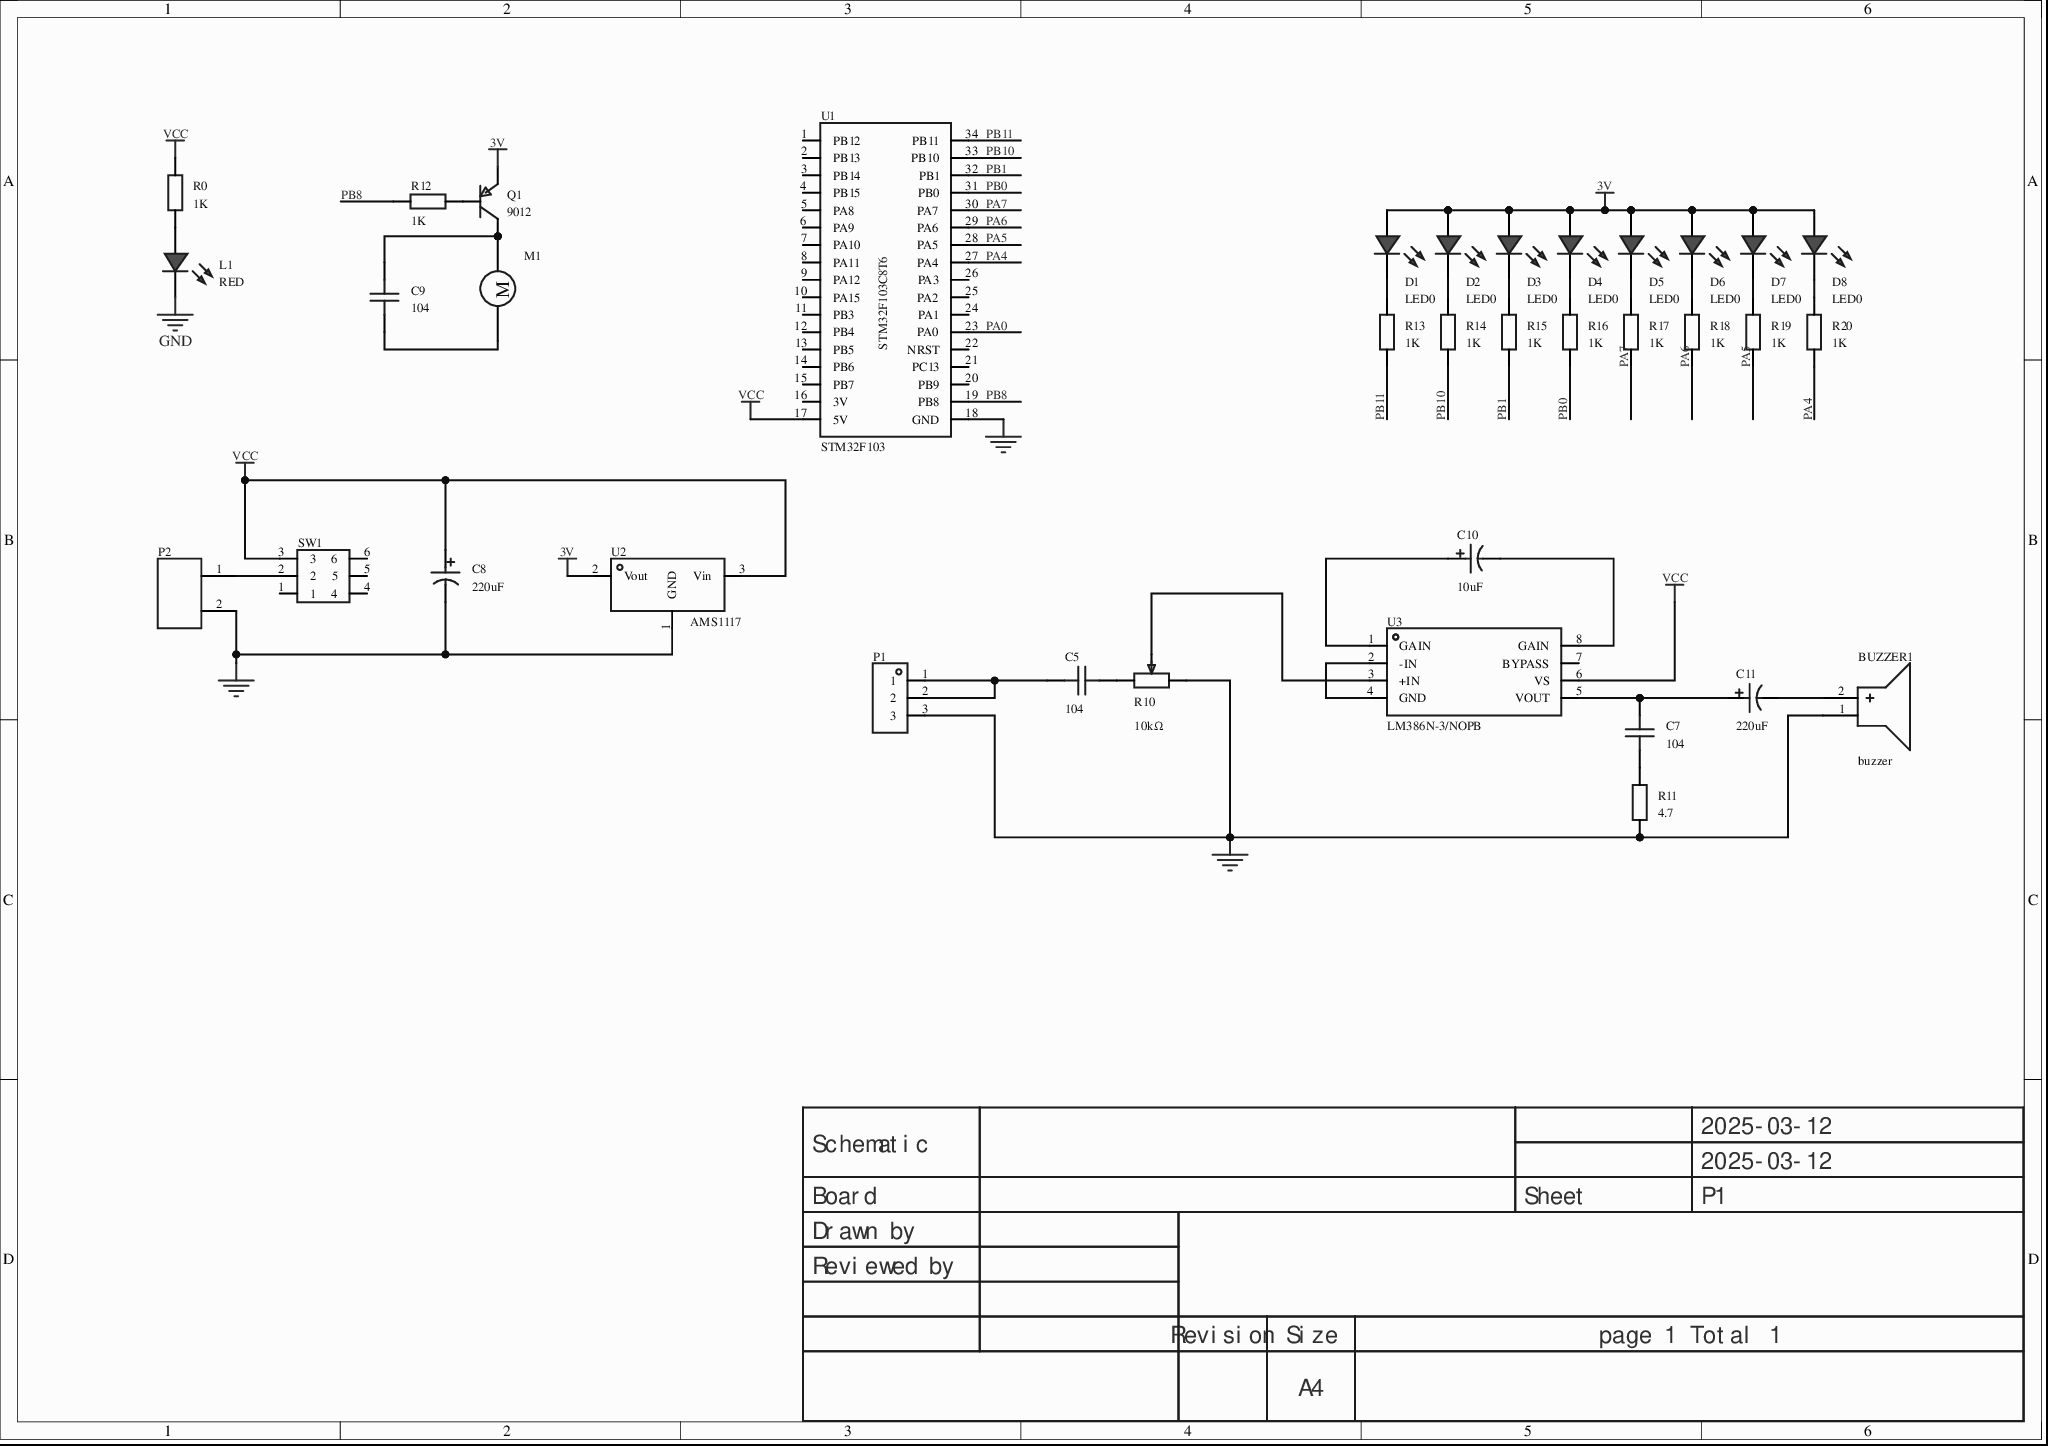
[diagram p0: MISC52120-3.schdoc]
# Altium project MISC52120-2.PrjPcb
1 sheet, 36 parts. Net scope: global (net labels, ports and power ports of the same name join across sheets).
Board file: MISC52120.pcbdoc

## Sheet MISC52120-3.schdoc
size 297 x 209 mm; Version: V1.0; @Project Name: MISC52120; @Page Count: 1; @Update Date: 2025-03-12; @Create Date: 2025-03-12; @Schematic Name: MISC52120; @Page No: 1; @Create Time: 16:08:51; @Update Time: 16:38:23; @Board Name: MISC52120

### Parts
BUZZER1  buzzer  [BUZ-TH_BD12.0-P6.00-D0.9-RD]
C5  104  [C0805]
C7  104  [C0805]
C8  220uF  [CAP-TH_BD6.3-P2.50-D1.0-FD]
C9  104  [C0805]
C10  10uF  [CAP-TH_BD5.0-P2.00-D0.8-FD]
C11  220uF  [CAP-TH_BD6.3-P2.50-D1.0-FD]
D1  LED0  [LED_TH-3mm]
D2  LED0  [LED_TH-3mm]
D3  LED0  [LED_TH-3mm]
D4  LED0  [LED_TH-3mm]
D5  LED0  [LED_TH-3mm]
D6  LED0  [LED_TH-3mm]
D7  LED0  [LED_TH-3mm]
D8  LED0  [LED_TH-3mm]
L1  RED  [LED_TH-3mm]
M1  Motor  [CONN-TH_2P-P5.08-WJ500V-5.08-2P]  (value not drawn)
P1  (no value)  [HDR-TH_3P-P2.54-V-M]
P2  DC005  [DC-IN-TH_DC005]  (value not drawn)
Q1  9012  [SOT-23-3_L2.9-W1.3-P1.90-LS2.4-BR]
R0  1K  [R0603]
R10  10kΩ  [R_3296]
R11  4.7  [R0603]
R12  1K  [R0603]
R13  1K  [R0603]
R14  1K  [R0603]
R15  1K  [R0603]
R16  1K  [R0603]
R17  1K  [R0603]
R18  1K  [R0603]
R19  1K  [R0603]
R20  1K  [R0603]
SW1  Switch  [SW-TH_SS-12D01-GX]  (value not drawn)
U1  STM32F103  [LQFP-48_L7.0-W7.0-P0.50-LS9.0-BL]
U2  AMS1117  [SOT-223-3_L6.5-W3.4-P2.30-LS7.0-BR]
U3  LM386N-3/NOPB  [DIP-8_L9.8-W6.6-P2.54-LS7.6-BL]

### Nets
3V: D1.1(C) D2.1(C) D3.1(C) D4.1(C) D5.1(C) D6.1(C) D7.1(C) D8.1(C) Q1.2(E) U2.2(Vout)
GND: BUZZER1.1(-) C8.2 L1.2(A) P1.3 P2.2 R10.1 R11.1 U1.18(GND) U2.1(GND)
VCC: C8.1 R0.2 SW1.3 U1.17(5V) U2.3(Vin) U3.6(VS)
PA0: U1.23(PA0)
PA4: R20.1 U1.27(PA4)
PA5: R19.1 U1.28(PA5)
PA6: R18.1 U1.29(PA6)
PA7: R17.1 U1.30(PA7)
PB0: R16.1 U1.31(PB0)
PB1: R15.1 U1.32(PB1)
PB8: R12.2 U1.19(PB8)
PB10: R14.1 U1.33(PB10)
PB11: R13.1 U1.34(PB11)
NetBUZZER1_2: BUZZER1.2(+) C11.2
NetC5_1: C5.1 R10.3
NetC5_2: C5.2 P1.1 P1.2
NetC7_1: C7.1 C11.1 U3.5(VOUT)
NetC7_2: C7.2 R11.2
NetC9_1: C9.1 M1.2
NetC9_2: C9.2 M1.1 Q1.3(C)
NetC10_1: C10.1 U3.1(GAIN)
NetC10_2: C10.2 U3.8(GAIN)
NetD1_2: D1.2(A) R13.2
NetD2_2: D2.2(A) R14.2
NetD3_2: D3.2(A) R15.2
NetD4_2: D4.2(A) R16.2
NetD5_2: D5.2(A) R17.2
NetD6_2: D6.2(A) R18.2
NetD7_2: D7.2(A) R19.2
NetD8_2: D8.2(A) R20.2
NetL1_1: L1.1(C) R0.1
NetP2_1: P2.1 SW1.2
NetQ1_1: Q1.1(B) R12.1
NetR10_2: R10.2 U3.3(+IN)
NetU3_2: U3.2(-IN) U3.4(GND)

Not connected (* = marked no-connect by the designer): SW1 1 4 5 6; U1 1(PB12) 2(PB13) 3(PB14) 4(PB15) 5(PA8) 6(PA9) 7(PA10) 8(PA11) 9(PA12) 10(PA15) 11(PB3) 12(PB4) 13(PB5) 14(PB6) 15(PB7) 16(3V) 20(PB9) 21(PC13) 22(NRST) 24(PA1) 25(PA2) 26(PA3); U3 7(BYPASS)

### Notes on the sheet
- 2025-03-12
- Schematic
- Board
- Sheet
- P1
- Drawn by
- Reviewed by
- Revision
- Size
- A4
- page 1 Total 1

### Library data of the parts
BUZZER1 = buzzer: AddInBom: yes; ModelId: af17e4151ed84fc2a628230bf2376363; ModelTransform: 472.44,472.176,0,270,0,0,0,0,-196.85; Symbol: BUZZER; Device: buzzer; LCSC Part Name: buzzer; SupplierPart: C9900014030; ManufacturerPart: buzzer; Supplier Footprint: buzzer; JLCPCB Part Class: Extended library; Supplier: LCSC; ConvertToPcb: yes; FootprintName: BUZ-TH_BD12.0-P6.00-D0.9-RD; ModelName: BUZ-TH_BD12.0-P6.00-D0.9-RD
C5 C7 C9 = CAP_0805: ConvertToPcb: yes; SymbolName: CapAcitance; ModelId: 1ba041120af144c991958decab20d241; ModelName: C0805_L2.0-W1.3-H1.3; ModelTransform: 78.74,51.181,0,0,0,0,0,0.0005,0; Value: 104; Device: CAP_0805; AddInBom: yes; Supplier Footprint: 0805; FootprintName: C0805
C8 C11 = EF227M010E05RR0VH4FP0: Capacitance: 220uF; tolerance: ±20%; rated voltage: 10V; ripple current: -; equivalent series resistance: -;; Manufacturer: CX(承兴); Symbol: 220uF 10Vblack gold 6.3*5; AddInBom: yes; ModelId: 0a4db4bf24b443b3be4905be97ff10c5; ModelTransform: 248.4247,247.99777,0,0,0,0,0,0,-137.795; φD: 6.3mm; L: 5mm; Lifetime @ Temp: 1000hrs@105℃; Device: EF227M010E05RR0VH4FP0; LCSC Part Name: 220uF ±20% 10V 黑; SupplierPart: C43330; ManufacturerPart: EF227M010E05RR0VH4FP0; Supplier Footprint: 插件,D6.3xL5mm; JLCPCB Part Class: Extended library; Datasheet: https://atta.szlcsc.com/upload/public/pdf/source/20211027/17061127B1D79C430F12717C63BD8A03.pdf; Supplier: LCSC; ConvertToPcb: yes; FootprintName: CAP-TH_BD6.3-P2.50-D1.0-FD; ModelName: CAP-TH_BD6.3-P2.50-D1.0-FD; Value: 220uF; Tolerance: ±20%; Rated Voltage: 10V; Ripple Current: -; Equivalent Series Resistance(ESR): -; Lead Spacing: 2.5mm; Operating Temperature: -40℃~+105℃
C10 = ERM1HM100D11OT: Capacitance: 10uF; tolerance: ±20%; rated voltage: 50V; ripple current: 90mA@100kHz; equivalent series resistance: -;; Manufacturer: AISHI(艾华集团); AddInBom: yes; ModelId: edeeed87cbc746108d01291548c38636; ModelName: CAP-TH_D5.0×H7.0×P2.0; ModelTransform: 197.091,196.7911,0,0,0,0,0,0,-137.795; φD: 5mm; L: 11mm; Lifetime @ Temp: 10000hrs@105℃; Symbol: ERM1HM100D11OT; Device: ERM1HM100D11OT; LCSC Part Name: 10uF ±20% 50V; SupplierPart: C106599; ManufacturerPart: ERM1HM100D11OT; Supplier Footprint: 插件,D5xL11mm; JLCPCB Part Class: Extended library; Datasheet: https://atta.szlcsc.com/upload/public/pdf/source/20190702/C401548_D47CA6D0010873F569B1039B34C05C69.pdf; Supplier: LCSC; ConvertToPcb: yes; FootprintName: CAP-TH_BD5.0-P2.00-D0.8-FD; Value: 10uF; Tolerance: ±20%; Rated Voltage: 50V; Ripple Current: 90mA@100kHz; Equivalent Series Resistance(ESR): -; Lead Spacing: 2mm
D1-D8 L1 = LED_TH-R_3mm: ConvertToPcb: yes; ModelId: a497c992633541038a38947cdc58012f; ModelName: LED-TH-3mm_R; ModelTransform: 141.274,153.327,0,0,0,0,-5.984,0,-137.795; Symbol: LED_TH-R; Device: LED_TH-R_3mm; AddInBom: yes; FootprintName: LED_TH-3mm; Supplier Footprint: 插件
M1 = Motor: AddInBom: yes; Device: Motor; ConvertToPcb: yes; SymbolName: Motor; FootprintName: CONN-TH_2P-P5.08-WJ500V-5.08-2P
P1 = HDR-M_2.54_1x3P: Symbol: PZ254V-11-03P_C2937625; ConvertToPcb: yes; ModelId: bb473b6d38ff42a99216a4fcdbdcc4cb; ModelName: HDR-TH_3P-P2.54-M-LI-1X3P; ModelTransform: 299.9994,100,0,0,0,0,0,0,-118.11; Device: HDR-M_2.54_1x3P; AddInBom: yes; SupplierPart: C2937625; Supplier Footprint: 插件; FootprintName: HDR-TH_3P-P2.54-V-M
P2 = DC005: Connector type: DC power socket; mounting: right-angle; contact inner diameter: 2mm; contact outer diameter: 6.3mm; rated current: 500mA; rated voltage: 30V; operating temperature range: -25℃~+70℃;; Manufacturer: SHOU HAN(首韩); Symbol: DC005_C431533; AddInBom: yes; ModelId: f168fe383f964e0ea2af0127ff6ac7b4; ModelTransform: 366.141,553.149,0,270,0,0,-141.734,88.583,-149.606; Device: DC005; LCSC Part Name: DC电源插座 内径:2mm 外径:6.3mm; SupplierPart: C431533; ManufacturerPart: DC005; Supplier Footprint: 插件; Datasheet: https://atta.szlcsc.com/upload/public/pdf/source/20190925/C431533_4751811035784AC1D38EBC85F7905E99.pdf; Supplier: LCSC; ConvertToPcb: yes; Connector Type: DC power socket; Mounting Style: Right-angle; Inside Contact Diameter: 2mm; Outside Contact Diameter: 6.3mm; Current Rating (Max): 500mA; Voltage Rating (Max): 30V; Operating Temperature Range: -25℃~+70℃; FootprintName: DC-IN-TH_DC005; ModelName: DC-IN-TH_DC005
Q1 = S9012 2T1(RANGE:200-350): Transistor type: PNP; collector current (Ic): 500mA; collector-emitter breakdown voltage (Vceo): 25V; power (Pd): 300mW; DC current gain (hFE@Ic,Vce): 120@50mA,1V;; Manufacturer: CJ(江苏长电/长晶); AddInBom: yes; ModelId: c62791f0466c4ae2a892c056b845b0ca; ModelName: SOT-23-3P_L2.9-W1.3-H1.0-LS2.4-P0.95; ModelTransform: 98.425,114.173,0,180,0,0,0.0005,-0.0005,0; Transition Frequency (fT): 150MHz; Collector Cut-Off Current (Icbo): 100nA; Collector-Emitter Saturation Voltage (VCE(sat)@Ic,Ib): 600mV@500mA,50mA; Symbol: S9012 2T1; Manufacturer Part: 9012; Device: S9012 2T1(RANGE:200-350); LCSC Part Name: PNP 电流:500mA 耐压:25V H档(200-350); SupplierPart: C8543; Supplier Footprint: SOT-23; JLCPCB Part Class: Basic library; Datasheet: https://atta.szlcsc.com/upload/public/pdf/source/20171228/C164889_15144412907211213892.pdf; Supplier: LCSC; ConvertToPcb: yes; FootprintName: SOT-23-3_L2.9-W1.3-P1.90-LS2.4-BR; Transistor Type: PNP; Collector Current (Ic): 500mA; Collector-Emitter Breakdown Voltage (Vceo): 25V; Power Dissipation (Pd): 300mW; DC Current Gain (hFE@Ic,Vce): 120@50mA,1V; Operating Temperature: -55℃~+150℃
R0 R11-R20 = Res_0603: ConvertToPcb: yes; SymbolName: Resistor; ModelId: fc143cca1e79419f9cd78b61e9279f08; ModelTransform: 31.8897,63.7794,0,90,0,0,0,0,0; Device: Res_0603; AddInBom: yes; Supplier Footprint: 0603; FootprintName: R0603; ModelName: R0603
  R0 R12-R20: Value: 1K
  R11: Value: 4.7
R10 = R_3296: ConvertToPcb: yes; ModelId: b182808559bb43bda9e7de64b64134cb; ModelName: 3296W; ModelTransform: 373.98,188.96,590.49,180,0,0,0,0,-140; Device: R_3296; AddInBom: yes; Supplier Footprint: 直插; SymbolName: R_3296; FootprintName: R_3296; Value: 10kΩ
SW1 = 开关: AddInBom: yes; ModelId: 46ec4e06866345239622c383c14b792d; ModelTransform: 346.456,153.543,0,0,0,0,-0.005,0,-169.291; Symbol: Switch; Device: Switch; LCSC Part Name: 开关; SupplierPart: C9900023015; ManufacturerPart: 开关; Supplier Footprint: SW-TH; JLCPCB Part Class: Extended library; Supplier: LCSC; ConvertToPcb: yes; FootprintName: SW-TH_SS-12D01-GX; ModelName: SW-TH_SS-12D01-GX
U1 = STM32F103C8T6: CPU core: ARM-M3; CPU max frequency: 72MHz; application field: -;; Manufacturer: ST(意法半导体); AddInBom: yes; Program Storage Size: 64KB; Program Memory Type: FLASH; Number of I/O: 37; ADC (Bit): 12bit; Low Voltage Detection Threshold: 2V~3.6V; ModelId: 093be70396ff421eb2cdb946d5311efc; ModelName: LQFP-48_L7.0-W7.0-H1.4-LS9.0-P0.50; ModelTransform: 354.331,354.331,0,0,0,0,0,0,0; Manufacturer Part: STM32F103; Symbol: STM32F103C8T6; Device: STM32F103C8T6; LCSC Part Name: 主流增强型ARM Cortex-M3 MCU，具有64 KB Flash、72 MHz CPU、电机控制、USB和CAN; SupplierPart: C8734; Supplier Footprint: LQFP-48(7x7); JLCPCB Part Class: Extended library; Datasheet: https://atta.szlcsc.com/upload/public/pdf/source/20220812/8363ACEC51AD55ECEB84799464F7CB85.pdf; Supplier: LCSC; ConvertToPcb: yes; CPU Core: ARM-M3; CPU Maximum Speed: 72MHz; Application Area: -; FootprintName: LQFP-48_L7.0-W7.0-P0.50-LS9.0-BL
U2 = AMS1117-3.3_C6186: Output type: fixed; operating voltage: -; output voltage: 3.3V; output current: 1A; PSRR: 72dB@(120Hz); output polarity: positive;; Manufacturer: AMS; AddInBom: yes; Voltage Dropout: 1.3V@(800mA); Number of Outputs: 1; ModelId: 925194bf9823436183a3e0b978a8d076; ModelName: SOT-223-4P_L6.5-W3.5-H1.6-LS7.0-P2.30; ModelTransform: 279.89794,255.905,0,180,0,0,-3.9385,-0.0005,0; Symbol: AMS1117-3.3; Manufacturer Part: AMS1117; Device: AMS1117-3.3_C6186; LCSC Part Name: 输出3.3V 1A; SupplierPart: C6186; Supplier Footprint: SOT-223; Datasheet: https://atta.szlcsc.com/upload/public/pdf/source/20180727/C6186_7A095716F0823C02F1997A905E26C086.pdf; Supplier: LCSC; ConvertToPcb: yes; Output Type: Fixed; Voltage - Supply: -; Output Voltage: 3.3V; Output Current: 1A; Power Supply Rejection Ratio (PSRR): 72dB@(120Hz); standby current: -; Noise: -; Features: Overcurrent protection (OCP); thermal shutdown (TSD); Operating Temperature: -; Output Configuration: Positive; FootprintName: SOT-223-3_L6.5-W3.4-P2.30-LS7.0-BR
U3 = LM386N-3/NOPB: Amplifier type: class AB amplifier; speaker channels: mono; output power: 700mWx1@8Ω;; Manufacturer: TI(德州仪器); AddInBom: yes; ModelId: db2af726fcec488f8bf8e467aca974b3; ModelName: DIP-8_L9.8-W6.6-H3.5-LS7.62-P2.54; ModelTransform: 385.826,311.8104,0,0,0,0,-1.693,0,-137.795; Supply Voltage: 4V~12V; Symbol: LM386N-3; Device: LM386N-3/NOPB; LCSC Part Name: 700mW单声道AB类音频功率放大器; SupplierPart: C139428; ManufacturerPart: LM386N-3/NOPB; Supplier Footprint: DIP-8; JLCPCB Part Class: Extended library; Supplier: LCSC; ConvertToPcb: yes; FootprintName: DIP-8_L9.8-W6.6-P2.54-LS7.6-BL; Type of Power Amplifier: Class AB amplifier; Speaker Channels: Mono; Output Power: 700mWx1@8Ω; Operating Temperature: 0℃~+70℃